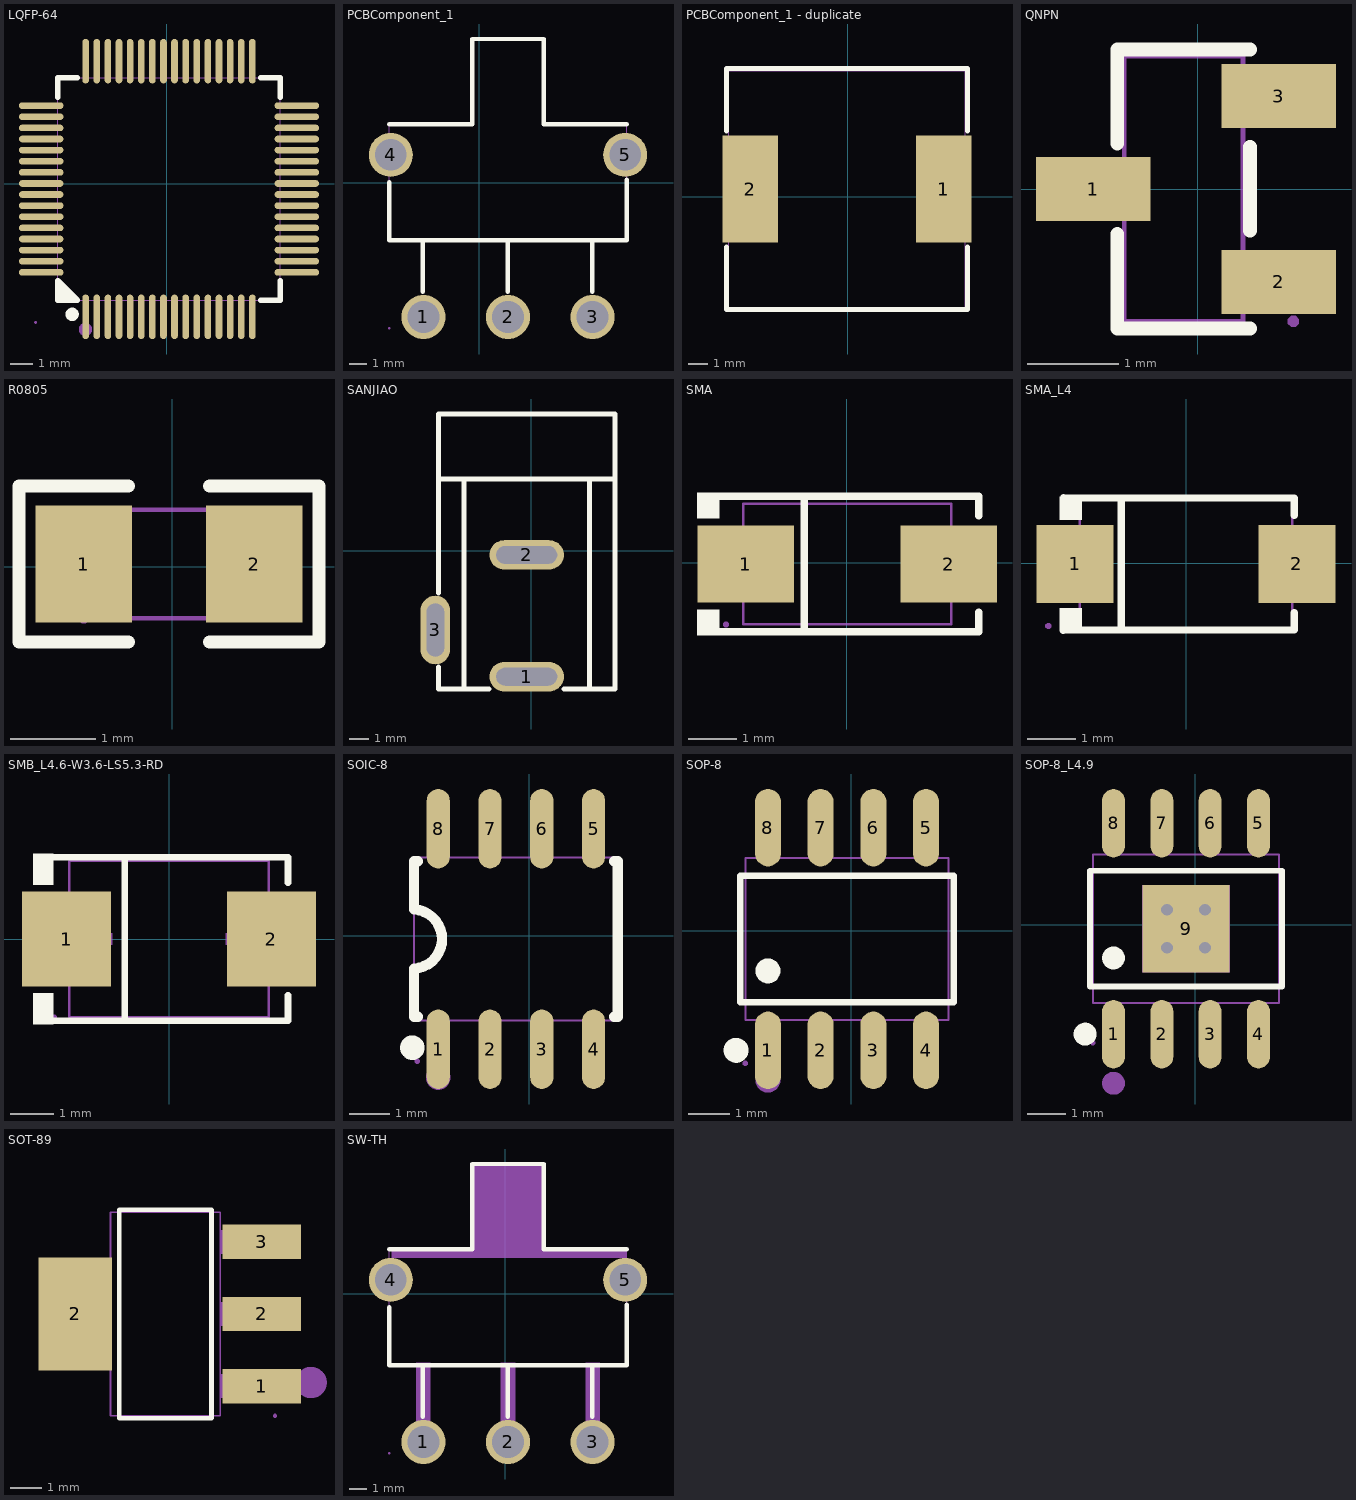
[diagram p0: the footprints below, top view; thin cyan lines are the x and y axes]
# Altium footprint library MISC82341-7.PcbLib: 30 footprints (part 2 of 2)
Each footprint in its own frame and in the unit in brackets; x right, y up, seen from the top. Pads: shape width x height; smd on the part's side, far side on the other; paste and mask are expansions set on the pad; w line width, h text height; cw(c..) or ccw(c..) is an arc to the next point about the centre after c.

## LQFP-64 [mm]
pads (64):
  oval 0.3x2 smd: 1(-3.639,-5.988) 2(-3.139,-5.988) 3(-2.639,-5.988) 4(-2.139,-5.988) 5(-1.639,-5.988) 6(-1.139,-5.988) 7(-0.639,-5.988) 8(-0.139,-5.988) 9(0.361,-5.988) 10(0.861,-5.988) 11(1.361,-5.988) 12(1.861,-5.988) 13(2.361,-5.988) 14(2.861,-5.988) 15(3.361,-5.988) 16(3.861,-5.988) 33(3.861,5.512) 34(3.361,5.512) 35(2.861,5.512) 36(2.361,5.512) 37(1.861,5.512) 38(1.361,5.512) 39(0.861,5.512) 40(0.361,5.512) 41(-0.139,5.512) 42(-0.639,5.512) 43(-1.139,5.512) 44(-1.639,5.512) 45(-2.139,5.512) 46(-2.639,5.512) 47(-3.139,5.512) 48(-3.639,5.512)
  oval 2x0.3 smd: 17(5.861,-3.988) 18(5.861,-3.488) 19(5.861,-2.988) 20(5.861,-2.488) 21(5.861,-1.988) 22(5.861,-1.488) 23(5.861,-0.988) 24(5.861,-0.488) 25(5.861,0.012) 26(5.861,0.512) 27(5.861,1.012) 28(5.861,1.512) 29(5.861,2.012) 30(5.861,2.512) 31(5.861,3.012) 32(5.861,3.512) 49(-5.639,3.512) 50(-5.639,3.012) 51(-5.639,2.512) 52(-5.639,2.012) 53(-5.639,1.512) 54(-5.639,1.012) 55(-5.639,0.512) 56(-5.639,0.012) 57(-5.639,-0.488) 58(-5.639,-0.988) 59(-5.639,-1.488) 60(-5.639,-1.988) 61(-5.639,-2.488) 62(-5.639,-2.988) 63(-5.639,-3.488) 64(-5.639,-3.988)
Top Overlay:
  region: -4.02,-5.238 -4.889,-4.369 -4.889,-5.238
  lines w0.254: -4.889,3.893 -4.889,4.762 -4.02,4.762 ; 4.242,-5.238 5.111,-5.238 5.111,-4.369 ; 4.242,4.762 5.111,4.762 5.111,3.893 ; -4.889,-4.369 -4.889,-4.369 ; -4.889,-4.369 -4.02,-5.238 -4.889,-5.238 -4.889,-4.369
  lines w0.3: -4.25,-5.728 ccw(c-4.249,-5.878) -4.248,-5.728
Mechanical 6:
  circle w0.3: c-3.649,-6.558 r0.15
Mechanical 15:
  drawing of 133 lines, arcs and shapes, not listed

## PCBComponent_1 [mm]
pads (5):
  round 2.5 hole 1.8: 1(-3.159,-7.63) 2(1.641,-7.63) 3(6.441,-7.63) 4(-5.009,1.57) 5(8.291,1.57)
Top Overlay:
  lines w0.254: -5.09,0.018 -5.09,-3.284 8.372,-3.284 8.372,0.145 ; -5.09,3.32 -0.391,3.32 -0.391,8.146 3.673,8.146 3.673,3.32 8.372,3.32 ; -3.194,-6.205 -3.194,-3.284 ; 1.632,-6.205 1.632,-3.284 ; 6.432,-6.205 6.432,-3.284
Mechanical 15:
  region: -5.049,-8.28 -5.049,-8.255 -5.084,-8.22 -5.134,-8.22 -5.169,-8.255 -5.169,-8.28 -5.169,-8.305 -5.134,-8.34 -5.084,-8.34 -5.049,-8.305
  region: -3.559,-6.98 -2.759,-6.98 -2.759,-8.28 -3.559,-8.28
  region: 6.041,-6.98 6.841,-6.98 6.841,-8.28 6.041,-8.28
  region: -5.109,2.195 -4.909,2.195 -4.909,0.945 -5.109,0.945
  region: 8.191,2.195 8.391,2.195 8.391,0.945 8.191,0.945
  region: 1.241,-6.98 2.041,-6.98 2.041,-8.28 1.241,-8.28
  lines w0.051: -5.109,-3.332 -5.109,3.268 -0.459,3.27 -0.459,8.096 3.741,8.096 3.741,3.27 8.391,3.268 8.391,-3.332 -5.109,-3.332

## PCBComponent_1 - duplicate [mm]
pads (2):
  rect 2.8x5.4 smd: 1(4.85,0.381) 2(-4.95,0.381)
Top Overlay:
  lines w0.254: -6.146,-2.55 -6.146,-5.715 6.046,-5.715 6.046,-2.55 ; -6.146,3.312 -6.146,6.477 6.046,6.477 6.046,3.312
Mechanical 15:
  region: 6.01,6.381 6.01,6.406 5.975,6.441 5.925,6.441 5.89,6.406 5.89,6.381 5.89,6.356 5.925,6.321 5.975,6.321 6.01,6.356
  region: 5.95,2.481 5.95,-1.719 3.95,-1.719 3.95,2.481
  region: -4.05,2.481 -4.05,-1.719 -6.05,-1.719 -6.05,2.481
  lines w0.051: -6.05,-5.619 -6.05,6.381 5.95,6.381 5.95,-5.619 -6.05,-5.619

## QNPN [mm]
pads (3):
  rect 1.25x0.7 smd: 1(-1.143,0) 2(0.889,-1.016) 3(0.889,1.016)
Top Overlay:
  lines w0.152: -0.879,-0.492 -0.879,-1.524 0.573,-1.524 ; -0.879,0.497 -0.879,1.528 0.573,1.528 ; 0.573,-0.453 0.573,0.458
Mechanical 6:
  circle w0.2: c1.307,-1.098 r0.1
Mechanical 15:
  region: 1.107,-1.448 1.107,-1.423 1.072,-1.388 1.022,-1.388 0.987,-1.423 0.987,-1.448 0.987,-1.473 1.022,-1.508 1.072,-1.508 1.107,-1.473
  region: 0.487,0.737 0.487,1.167 0.757,1.167 0.757,0.737
  region: 0.747,0.737 0.747,1.167 1.047,1.167 1.047,0.737
  region: 0.487,-1.163 0.487,-0.733 0.757,-0.733 0.757,-1.163
  region: 0.747,-1.163 0.747,-0.733 1.047,-0.733 1.047,-1.163
  region: -1.063,-0.213 -1.063,0.217 -0.793,0.217 -0.793,-0.213
  region: -1.353,-0.213 -1.353,0.217 -1.053,0.217 -1.053,-0.213
  lines w0.051: -0.803,-1.448 -0.803,1.452 0.497,1.452 0.497,-1.448 -0.803,-1.448

## R0805 [mm]
pads (2):
  rect 1.133x1.377 smd paste-100 mask+0.051: 1(-1.04,0.031) 2(0.96,0.031)
Top Overlay:
  lines w0.152: -0.516,-0.886 -1.801,-0.886 -1.801,0.948 -0.516,0.948 ; 0.437,-0.886 1.721,-0.886 1.721,0.948 0.437,0.948
Top Paste:
  region: -1.74,-0.609 -1.74,0.671 -1.69,0.721 -0.54,0.721 -0.49,0.671 -0.485,0.261 -0.935,0.261 -0.935,-0.189 -0.495,-0.189 -0.49,-0.609 -0.54,-0.659 -1.69,-0.659
  region: 0.41,-0.609 0.41,-0.189 0.855,-0.189 0.855,0.261 0.415,0.261 0.41,0.671 0.46,0.721 1.61,0.721 1.66,0.671 1.66,-0.609 1.61,-0.659 0.46,-0.659
Mechanical 15:
  region: -1.04,-0.606 -1.04,0.669 -0.64,0.669 -0.64,-0.606
  region: 0.96,-0.606 0.96,0.669 0.56,0.669 0.56,-0.606
  region: -0.98,-0.606 -0.98,-0.582 -1.015,-0.546 -1.065,-0.546 -1.1,-0.582 -1.1,-0.606 -1.1,-0.631 -1.065,-0.666 -1.015,-0.666 -0.98,-0.631
  lines w0.051: -1.04,-0.606 -1.04,0.669 0.96,0.669 0.96,-0.606 -1.04,-0.606

## SANJIAO [mm]
pads (3):
  oval 3.8x1.5 hole 0.9 slot 3.1 at 0 deg paste+0 mask+0.051: 1(-0.226,-6.422) 2(-0.226,-0.222)
  oval 1.5x3.5 hole 0.9 slot 2.7 at 90 deg paste+0 mask+0.051: 3(-4.876,-4.044)
Top Overlay:
  lines w0.254: -4.726,-5.928 -4.726,-7.044 -2.134,-7.044 ; -4.726,-2.16 -4.726,6.956 4.274,6.956 4.274,-7.044 1.682,-7.044 ; -4.726,3.656 4.274,3.656 ; -3.426,-7.044 -3.426,3.576 ; 2.974,-7.044 2.974,3.576
Mechanical 15:
  lines w0.003: 0.357,-0.318 0.358,-0.317

## SMA [mm]
pads (2):
  rect 2x1.593 smd: 1(-2.087,-0.023) 2(2.113,-0.023)
Top Overlay:
  region: -2.637,-1.5 -2.637,-0.972 -3.094,-0.972 -3.094,-1.5
  region: -2.637,1.455 -2.637,0.926 -3.094,0.926 -3.094,1.455
  lines w0.152: -2.713,-1.424 2.74,-1.424 2.74,-1.023 ; -2.713,1.378 2.74,1.378 2.74,0.977 ; -0.873,-1.424 -0.873,1.378
Mechanical 6:
  region: 2.166,-0.685 2.166,0.64 1.968,0.64 1.968,-0.685
  region: 2.465,-0.122 2.465,0.076 1.67,0.076 1.67,-0.122
  region: -2.438,-0.122 -2.438,0.076 -1.643,0.076 -1.643,-0.122
Mechanical 15:
  region: 1.32,-0.748 1.32,0.702 2.52,0.702 2.52,-0.748
  region: -1.294,0.702 -1.294,-0.748 -2.494,-0.748 -2.494,0.702
  region: -2.433,-1.273 -2.433,-1.248 -2.469,-1.213 -2.518,-1.213 -2.553,-1.248 -2.553,-1.273 -2.553,-1.298 -2.518,-1.333 -2.469,-1.333 -2.433,-1.298
  lines w0.051: -2.137,-1.273 2.163,-1.273 2.163,1.227 -2.137,1.227 -2.137,-1.273

## SMA_L4 [mm]
pads (2):
  rect 1.6x1.62 smd: 1(-2.301,-0.011) 2(2.299,-0.011)
Top Overlay:
  region: -2.16,1.386 -2.16,0.908 -2.617,0.908 -2.617,1.386
  region: -2.16,-1.408 -2.16,-0.931 -2.617,-0.931 -2.617,-1.408
  lines w0.152: -2.544,-1.383 2.234,-1.375 ; -2.541,1.363 2.249,1.352 ; -1.34,-1.375 -1.34,1.352 ; 2.246,-1.375 2.246,-1.024 ; 2.246,1.002 2.246,1.352
Mechanical 6:
  region: -2.433,-0.108 -2.433,0.085 -1.66,0.085 -1.66,-0.108
  region: 2.431,-0.108 2.431,0.085 1.659,0.085 1.659,-0.108
  region: 2.141,-0.655 2.141,0.632 1.948,0.632 1.948,-0.655
Mechanical 15:
  region: -2.794,-1.299 -2.794,-1.274 -2.829,-1.239 -2.879,-1.239 -2.914,-1.274 -2.914,-1.299 -2.914,-1.324 -2.879,-1.359 -2.829,-1.359 -2.794,-1.324
  region: 2.666,0.739 2.666,-0.761 1.566,-0.761 1.566,0.739
  region: -2.668,-0.761 -2.668,0.739 -1.568,0.739 -1.568,-0.761
  lines w0.051: -2.201,-1.411 2.199,-1.411 2.199,1.389 -2.201,1.389 -2.201,-1.411

## SMB_L4.6-W3.6-LS5.3-RD [mm]
pads (2):
  rect 2.047x2.192 smd: 1(-2.361,0) 2(2.361,0)
Top Overlay:
  region: -2.668,1.962 -2.668,1.249 -3.125,1.249 -3.125,1.962
  region: -2.668,-1.962 -2.668,-1.249 -3.125,-1.249 -3.125,-1.962
  lines w0.152: -2.744,-1.886 2.744,-1.886 2.744,-1.299 ; -2.744,1.886 2.744,1.886 2.744,1.299 ; -1.016,-1.886 -1.016,1.886
Mechanical 6:
  region: -2.396,-0.136 -2.396,0.136 -1.31,0.136 -1.31,-0.136
  region: 2.396,-0.136 2.396,0.136 1.31,0.136 1.31,-0.136
  region: 1.989,-0.905 1.989,0.905 1.717,0.905 1.717,-0.905
Mechanical 15:
  region: -2.649,-1.015 -2.649,1.015 -1.509,1.015 -1.509,-1.015
  region: 2.649,-1.015 2.649,1.015 1.509,1.015 1.509,-1.015
  region: -2.59,-1.8 -2.59,-1.775 -2.625,-1.74 -2.674,-1.74 -2.709,-1.775 -2.709,-1.8 -2.709,-1.825 -2.674,-1.86 -2.625,-1.86 -2.59,-1.825
  lines w0.051: -2.3,-1.8 -2.3,1.8 2.3,1.8 2.3,-1.8 -2.3,-1.8

## SOIC-8 [mm]
pads (8):
  oval 0.568x1.95 smd: 1(-2.238,-2.788) 2(-0.968,-2.788) 3(0.302,-2.788) 4(1.572,-2.788) 5(1.572,2.622) 6(0.302,2.622) 7(-0.968,2.622) 8(-2.238,2.622)
Top Overlay:
  circle w0.3: c-2.873,-2.75 r0.15
  lines w0.254: -2.833,0.643 -2.833,1.417 -2.833,1.822 -2.742,1.822 ; -2.828,0.643 cw(c-2.873,-0.083) -2.833,-0.81 -2.833,-1.583 -2.833,-1.988 -2.742,-1.988 ; 2.075,-1.988 2.167,-1.988 2.167,-1.583 2.167,1.417 2.167,1.822 2.075,1.822
Mechanical 6:
  circle w0.3: c-2.238,-3.483 r0.15
Mechanical 15:
  region: -2.443,-3.083 -2.443,-2.248 -2.033,-2.248 -2.033,-3.083
  region: -2.443,-2.258 -2.443,-2.023 -2.033,-2.023 -2.033,-2.258
  region: -1.173,-3.083 -1.173,-2.248 -0.763,-2.248 -0.763,-3.083
  region: -1.173,-2.258 -1.173,-2.023 -0.763,-2.023 -0.763,-2.258
  region: 0.097,-3.083 0.097,-2.248 0.507,-2.248 0.507,-3.083
  region: 0.097,-2.258 0.097,-2.023 0.507,-2.023 0.507,-2.258
  region: 1.367,-3.083 1.367,-2.248 1.777,-2.248 1.777,-3.083
  region: 1.367,-2.258 1.367,-2.023 1.777,-2.023 1.777,-2.258
  region: -2.443,2.082 -2.443,2.917 -2.033,2.917 -2.033,2.082
  region: -2.443,1.857 -2.443,2.092 -2.033,2.092 -2.033,1.857
  region: -1.173,2.082 -1.173,2.917 -0.763,2.917 -0.763,2.082
  region: -1.173,1.857 -1.173,2.092 -0.763,2.092 -0.763,1.857
  region: 0.097,2.082 0.097,2.917 0.507,2.917 0.507,2.082
  region: 0.097,1.857 0.097,2.092 0.507,2.092 0.507,1.857
  region: 1.367,2.082 1.367,2.917 1.777,2.917 1.777,2.082
  region: 1.367,1.857 1.367,2.092 1.777,2.092 1.777,1.857
  region: -2.694,-3.083 -2.694,-3.058 -2.729,-3.023 -2.778,-3.023 -2.813,-3.058 -2.813,-3.083 -2.813,-3.108 -2.778,-3.143 -2.729,-3.143 -2.694,-3.108
  lines w0.051: -2.833,-2.083 2.167,-2.083 2.167,1.917 -2.833,1.917 -2.833,-2.083

## SOP-8 [mm]
pads (8):
  oval 0.63x1.865 smd: 1(-2.004,-2.878) 2(-0.734,-2.878) 3(0.536,-2.878) 4(1.806,-2.878) 5(1.806,2.487) 6(0.536,2.487) 7(-0.734,2.487) 8(-2.004,2.487)
Top Overlay:
  circle w0.3: c-2.004,-0.964 r0.15
  circle w0.3: c-2.771,-2.878 r0.15
  lines w0.152: -2.675,-1.716 -2.675,1.326 2.478,1.326 2.478,-1.716 -2.675,-1.716
Mechanical 6:
  circle w0.3: c-2.004,-3.595 r0.15
Mechanical 15:
  region: -2.489,-3.195 -2.489,-3.17 -2.524,-3.135 -2.573,-3.135 -2.609,-3.17 -2.609,-3.195 -2.609,-3.22 -2.573,-3.255 -2.524,-3.255 -2.489,-3.22
  region: 1.596,1.745 1.596,1.98 2.016,1.98 2.016,1.745
  region: 1.596,1.97 1.596,2.805 2.016,2.805 2.016,1.97
  region: 0.326,1.745 0.326,1.98 0.746,1.98 0.746,1.745
  region: 0.326,1.97 0.326,2.805 0.746,2.805 0.746,1.97
  region: -0.944,1.745 -0.944,1.98 -0.524,1.98 -0.524,1.745
  region: -0.944,1.97 -0.944,2.805 -0.524,2.805 -0.524,1.97
  region: -2.214,1.745 -2.214,1.98 -1.794,1.98 -1.794,1.745
  region: -2.214,1.97 -2.214,2.805 -1.794,2.805 -1.794,1.97
  region: 1.596,-2.37 1.596,-2.135 2.016,-2.135 2.016,-2.37
  region: 1.596,-3.195 1.596,-2.36 2.016,-2.36 2.016,-3.195
  region: 0.326,-2.37 0.326,-2.135 0.746,-2.135 0.746,-2.37
  region: 0.326,-3.195 0.326,-2.36 0.746,-2.36 0.746,-3.195
  region: -0.944,-2.37 -0.944,-2.135 -0.524,-2.135 -0.524,-2.37
  region: -0.944,-3.195 -0.944,-2.36 -0.524,-2.36 -0.524,-3.195
  region: -2.214,-2.37 -2.214,-2.135 -1.794,-2.135 -1.794,-2.37
  region: -2.214,-3.195 -2.214,-2.36 -1.794,-2.36 -1.794,-3.195
  lines w0.051: -2.549,-2.145 -2.549,1.755 2.351,1.755 2.351,-2.145 -2.549,-2.145

## SOP-8_L4.9 [mm]
pads (9):
  oval 0.6x1.8 smd: 1(-2.151,-2.876) 2(-0.881,-2.876) 3(0.389,-2.876) 4(1.659,-2.876) 5(1.659,2.669) 6(0.389,2.669) 7(-0.881,2.669) 8(-2.151,2.669)
  rect 2.29x2.29 smd: 9(-0.246,-0.104)
via 0.254,0.396 diameter 0.61 hole 0.305
via 0.254,-0.604 diameter 0.61 hole 0.305
via -0.746,-0.604 diameter 0.61 hole 0.305
via -0.746,0.396 diameter 0.61 hole 0.305
Top Overlay:
  circle w0.3: c-2.898,-2.876 r0.15
  circle w0.3: c-2.151,-0.873 r0.15
  lines w0.152: -2.773,-1.625 2.28,-1.625 2.28,1.418 -2.773,1.418 -2.773,-1.625
Mechanical 6:
  circle w0.3: c-2.151,-4.168 r0.15
Mechanical 15:
  region: -1.391,-1.249 -1.391,1.041 0.899,1.041 0.899,-1.249
  region: 1.449,2.071 1.449,1.836 1.869,1.836 1.869,2.071
  region: 1.449,2.896 1.449,2.061 1.869,2.061 1.869,2.896
  region: 0.179,2.071 0.179,1.836 0.599,1.836 0.599,2.071
  region: 0.179,2.896 0.179,2.061 0.599,2.061 0.599,2.896
  region: -1.091,2.071 -1.091,1.836 -0.671,1.836 -0.671,2.071
  region: -1.091,2.896 -1.091,2.061 -0.671,2.061 -0.671,2.896
  region: -2.361,2.071 -2.361,1.836 -1.941,1.836 -1.941,2.071
  region: -2.361,2.896 -2.361,2.061 -1.941,2.061 -1.941,2.896
  region: 1.449,-2.279 1.449,-2.044 1.869,-2.044 1.869,-2.279
  region: 1.449,-3.104 1.449,-2.269 1.869,-2.269 1.869,-3.104
  region: 0.179,-2.279 0.179,-2.044 0.599,-2.044 0.599,-2.279
  region: 0.179,-3.104 0.179,-2.269 0.599,-2.269 0.599,-3.104
  region: -1.091,-2.279 -1.091,-2.044 -0.671,-2.044 -0.671,-2.279
  region: -1.091,-3.104 -1.091,-2.269 -0.671,-2.269 -0.671,-3.104
  region: -2.361,-2.279 -2.361,-2.044 -1.941,-2.044 -1.941,-2.279
  region: -2.361,-3.104 -2.361,-2.269 -1.941,-2.269 -1.941,-3.104
  region: -2.636,-3.104 -2.636,-3.079 -2.672,-3.044 -2.721,-3.044 -2.756,-3.079 -2.756,-3.104 -2.756,-3.129 -2.721,-3.164 -2.672,-3.164 -2.636,-3.129
  lines w0.051: -2.696,-2.054 2.204,-2.054 2.204,1.846 -2.696,1.846 -2.696,-2.054

## SOT-89 [mm]
pads (4):
  rect 2.5x1.1 smd: 1(-27.355,-14.485) 2(-27.355,-12.185) 3(-27.355,-9.885)
  rect 2.34x3.6 smd: 2(-33.294,-12.185)
Top Overlay:
  lines w0.152: -31.896,-15.511 -28.953,-15.511 -28.953,-8.859 -31.896,-8.859 -31.896,-15.511
Mechanical 6:
  circle w0.5: c-25.773,-14.373 r0.25
Mechanical 15:
  region: -28.685,-10.26 -28.685,-9.51 -27.665,-9.51 -27.665,-10.26
  region: -27.675,-10.26 -27.675,-9.51 -26.925,-9.51 -26.925,-10.26
  region: -28.685,-12.56 -28.685,-11.81 -27.665,-11.81 -27.665,-12.56
  region: -27.675,-12.56 -27.675,-11.81 -26.925,-11.81 -26.925,-12.56
  region: -28.685,-14.86 -28.685,-14.11 -27.665,-14.11 -27.665,-14.86
  region: -27.675,-14.86 -27.675,-14.11 -26.925,-14.11 -26.925,-14.86
  region: -33.185,-13.685 -33.185,-10.685 -32.165,-10.685 -32.165,-13.685
  region: -33.925,-13.685 -33.925,-10.685 -33.175,-10.685 -33.175,-13.685
  region: -26.864,-15.435 -26.864,-15.41 -26.9,-15.375 -26.949,-15.375 -26.984,-15.41 -26.984,-15.435 -26.984,-15.46 -26.949,-15.495 -26.9,-15.495 -26.864,-15.46
  lines w0.051: -32.175,-15.435 -28.675,-15.435 -28.675,-8.935 -32.175,-8.935 -32.175,-15.435

## SW-TH [mm]
pads (5):
  round 2.5 hole 1.8: 1(-4.647,-8.402) 2(0.153,-8.402) 3(4.953,-8.402) 4(-6.497,0.798) 5(6.803,0.798)
Top Overlay:
  lines w0.254: -6.578,-0.754 -6.578,-4.056 6.884,-4.056 6.884,-0.627 ; -6.578,2.548 -1.879,2.548 -1.879,7.374 2.185,7.374 2.185,2.548 6.884,2.548 ; -4.682,-6.977 -4.682,-4.056 ; 0.144,-6.977 0.144,-4.056 ; 4.944,-6.977 4.944,-4.056
Mechanical 6:
  region: -1.752,7.247 -1.752,2.421 2.058,2.421 2.058,7.247
  region: -6.451,2.421 6.884,2.421 6.884,2.04 -6.451,2.04
Mechanical 15:
  region: -6.537,-9.052 -6.537,-9.027 -6.572,-8.992 -6.622,-8.992 -6.657,-9.027 -6.657,-9.052 -6.657,-9.077 -6.622,-9.112 -6.572,-9.112 -6.537,-9.077
  region: -5.047,-7.752 -4.247,-7.752 -4.247,-9.052 -5.047,-9.052
  region: 4.553,-7.752 5.353,-7.752 5.353,-9.052 4.553,-9.052
  region: -6.597,1.423 -6.397,1.423 -6.397,0.173 -6.597,0.173
  region: 6.703,1.423 6.903,1.423 6.903,0.173 6.703,0.173
  region: -0.247,-7.752 0.553,-7.752 0.553,-9.052 -0.247,-9.052
  region: 4.553,-3.902 5.353,-3.902 5.353,-9.052 4.553,-9.052
  region: -0.247,-3.902 0.553,-3.902 0.553,-9.052 -0.247,-9.052
  region: -5.047,-3.902 -4.247,-3.902 -4.247,-9.052 -5.047,-9.052
  lines w0.051: -6.597,-4.104 -6.597,2.496 -1.947,2.498 -1.947,7.324 2.253,7.324 2.253,2.498 6.903,2.496 6.903,-4.104 -6.597,-4.104